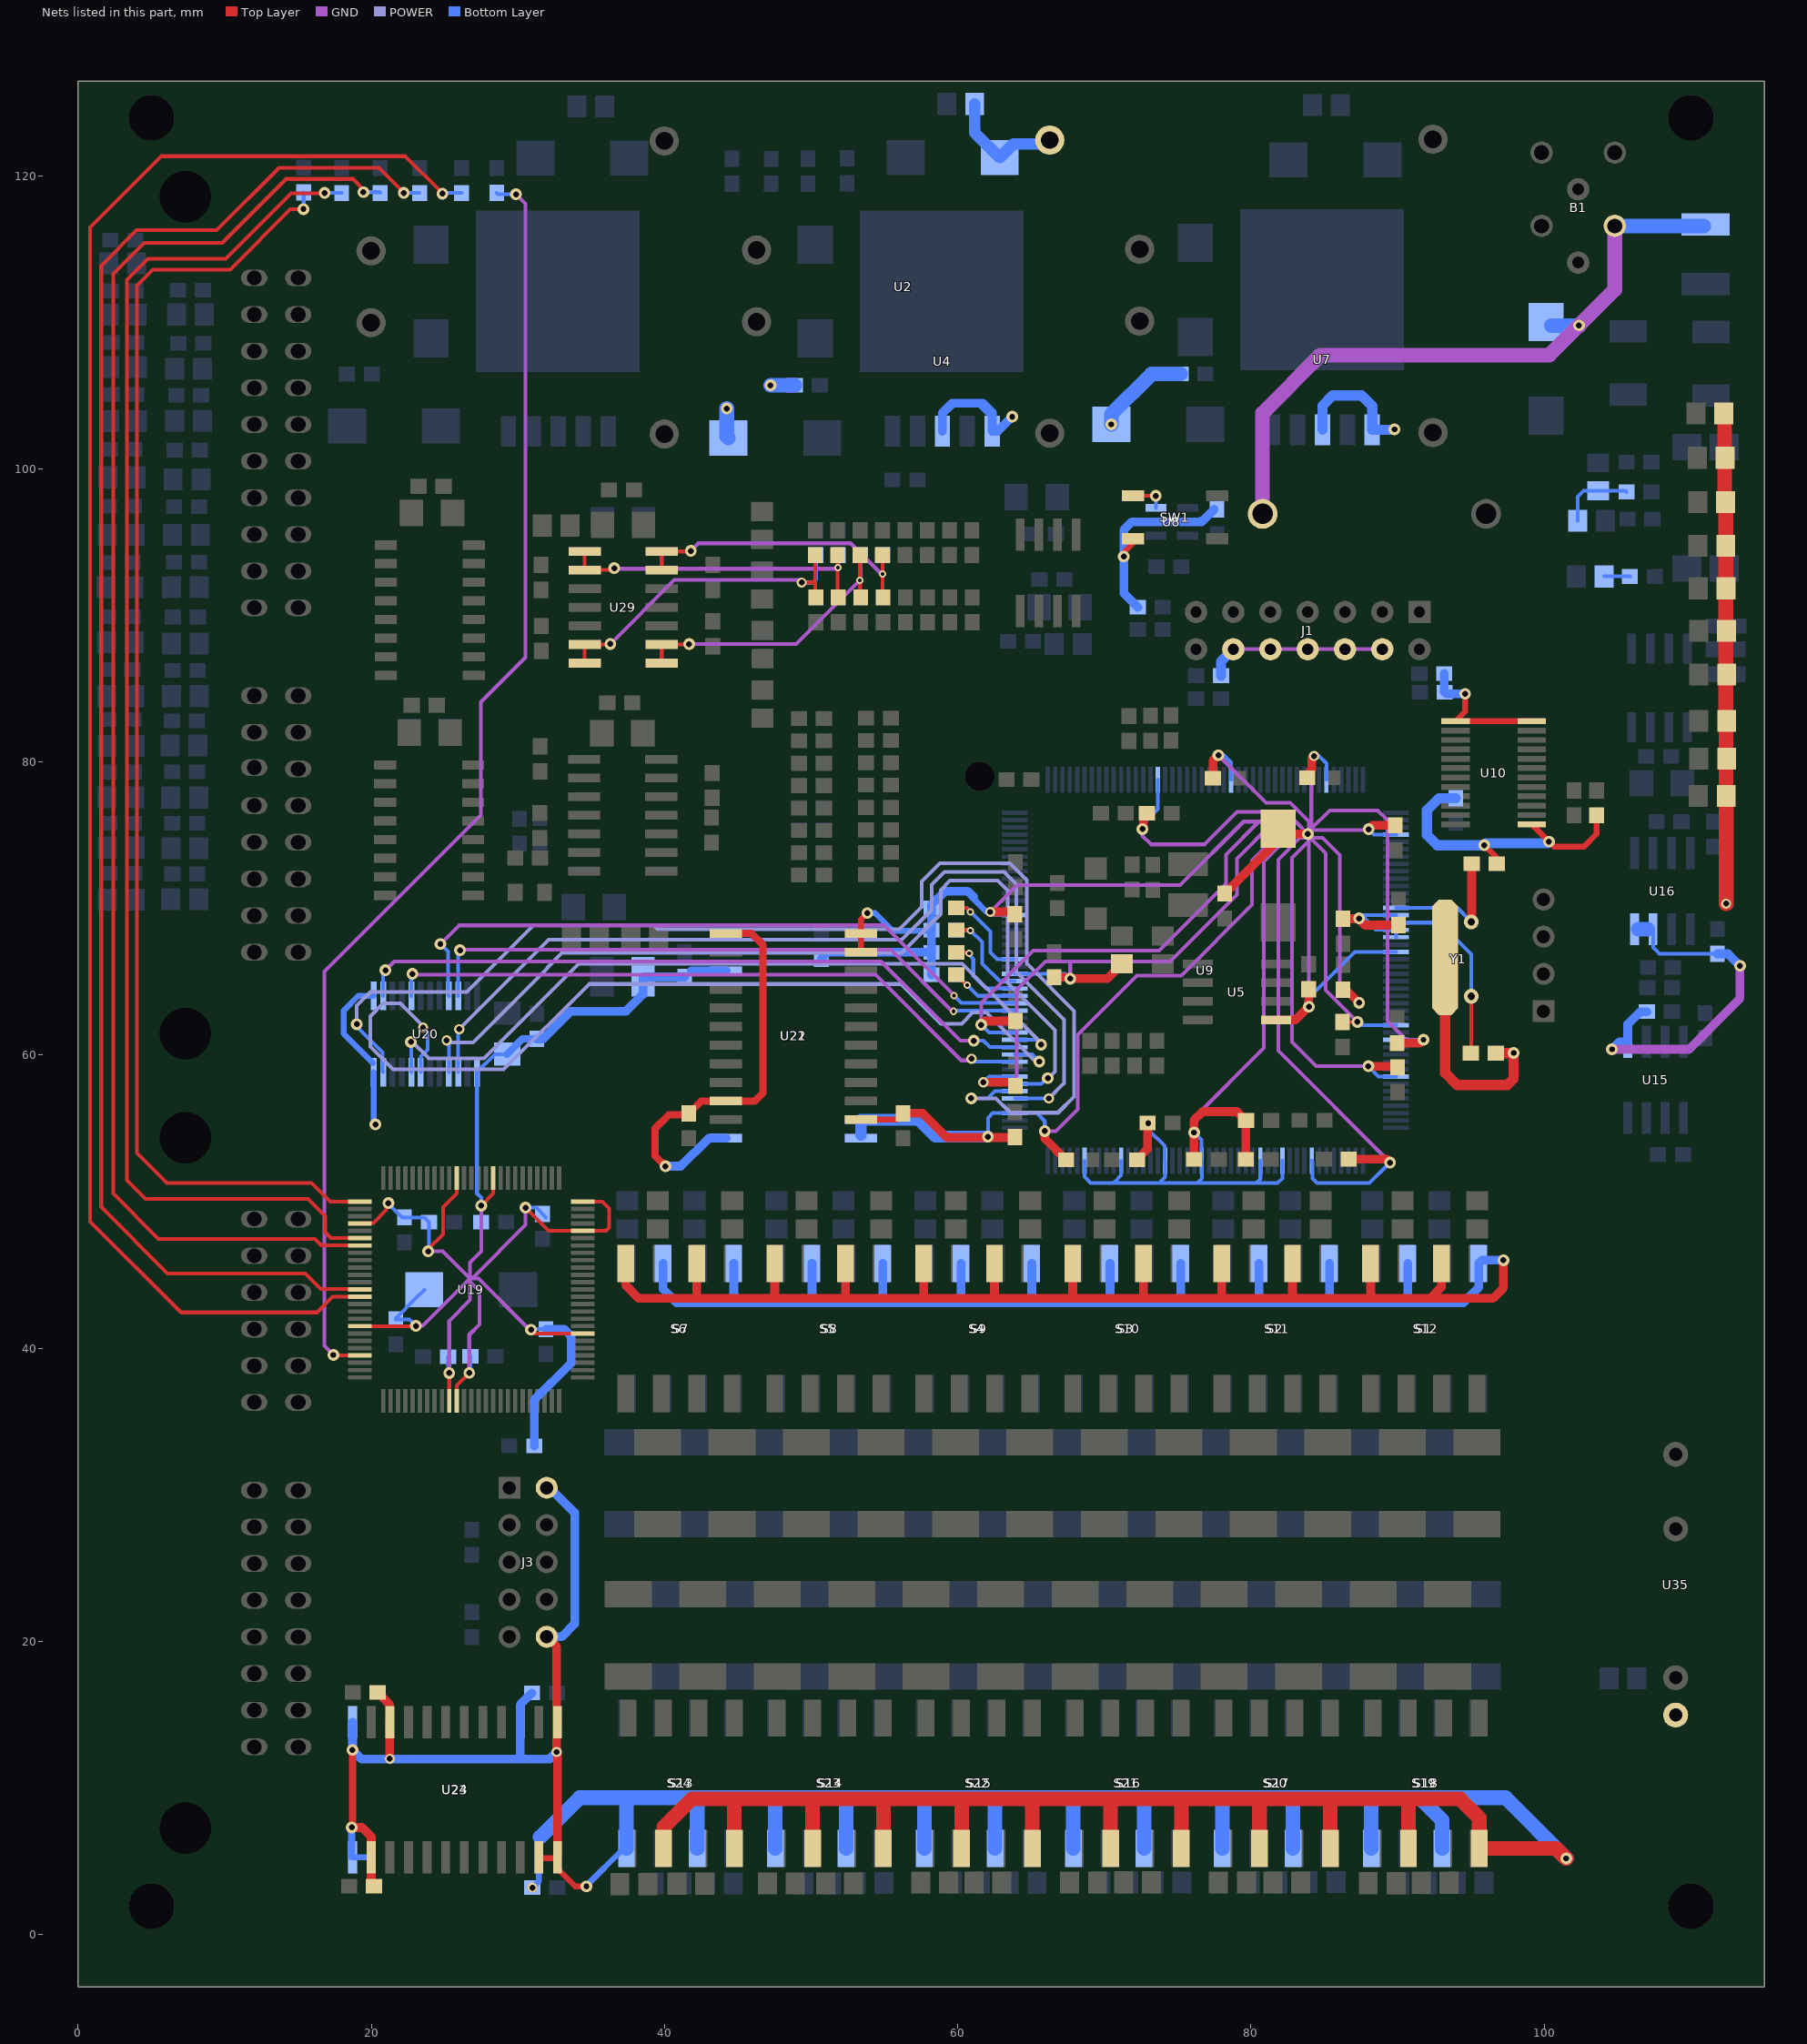
[diagram p0: the nets of this part, all layers, seen from the top]
# Altium PCB MISC86180.PCBDOC (part 7 of 9)
Units mm, origin at the board's own origin, x right, y up, seen from the top; angles counter-clockwise.
Board outline 115 x 130 mm, 4 copper layers (Top Layer, GND, POWER, Bottom Layer); 475 components, 355 nets, 1755 pads, 459 vias.

## Via types
v1: diameter 0.8, hole 0.4, Top Layer to Bottom Layer, 339 vias
v2: diameter 0.7, hole 0.4, Top Layer to Bottom Layer, 83 vias
v3: diameter 0.5, hole 0.254, Top Layer to Bottom Layer, 37 vias

## Nets (pads, with @x,y where several pads share a name; then routed paths per layer and width w, separated by ;. In a path a pad name is that pad's centre, name@x,y a point inside that pad or via, vN(x,y) a via of type N, cw(c..) or ccw(c..) an arc to the next point about the centre after c; other vN are vias at no path point) (continued)
GNDD: C6.2 C7.1 C11.2 C12.1 C13.2 C14.1 C17.2 C18.1 C19.1 C20.1 C21.1 C22.1 C23.1 C24.1 C25.1 C26.1 C27.1 C28.1 C29.1 C30.1 C31.1 C32.1 C33.1 C34.1 C35.1 C36.1 C37.1 C38.1 C39.1 C40.1 C41.1 C42.1 C52.1 C53.1 C54.1 C55.1 C56.1 C57.1 C67.1 C68.1 C81.2 C82.1 C83.1 C84.1 C85.1 C86.1 C87.1 C88.1 C89.1 C90.1 C91.1 C92.1 C93.1 C94.1 C95.1 C96.1 C97.1 C98.1 C99.1 D1.2 D2.2 D3.2 D4.2 D5.2 D6.2 D7.2 D8.2 D9.2 D10.2 J1.4 J1.6 J1.8 J1.10 J1.12 J3.2 J3.10 L2.1 R4.1 R5.1 R14.1 R83.1 R87.2 R89.2 R91.2 R93.2 S1.2 S1.4 S2.2 S2.4 S3.2 S3.4 S4.2 S4.4 S5.2 S5.4 S6.2 S6.4 S7.2 S7.4 S8.2 S8.4 S9.2 S9.4 S10.2 S10.4 S11.2 S11.4 S12.2 S12.4 S13.2 S13.4 S14.2 S14.4 S15.2 S15.4 S16.2 S16.4 S17.2 S17.4 S18.2 S18.4 S19.2 S19.4 S20.2 S20.4 S21.2 S21.4 S22.2 S22.4 S23.2 S23.4 S24.2 S24.4 SW1.2 U2.4 U4.1 U4.3 U5.1 U7.1 U7.3 U8.2 U9.3 U9.8 U9.14 U9.22 U9.30 U9.60 U9.70 U9.83 U9.92 U9.103 U9.105 U9.106 U9.108 U9.118 U9.120 U9.125 U9.140 U9.144 U9.147 U9.155 U9.160 U9.166 U9.171 U10.1 U10.12 U10.13 U15.5 U16.3 U16.4 U19.10 U19.11 U19.32 U19.46 U19.50 U19.60 U19.65 U19.79 U19.93 U20.1 U20.12 U20.13 U21.2 U21.11 U21.12 U21.13 U21.22 U22.2 U22.11 U22.12 U22.13 U22.22 U23.2 U23.11 U23.12 U23.13 U23.22 U24.2 U24.11 U24.12 U24.13 U24.22 U35.1 Y1.3 | length 1278
  Top Layer w0.254: U19.93@19.216,41.514 v1@23.024,41.514 ; U19.79@19.216,48.514 19.261,48.559 20.142,48.559 21.02,49.437 21.02,49.79 21.14,49.91 v1(21.17,49.91) ; U23.2@19.98,5.283 U23.2@19.989,5.292 ; U23.22@21.259,14.492 21.259,15.681 21.268,15.69 21.259,15.699 ; v1(23.88,46.62) 23.88,46.77 24.89,47.78 24.89,49.63 25.816,50.556 U19.65@25.816,51.614 ; U19.10@25.316,36.414 v1(25.316,38.314) ; U19.11@25.816,36.414 25.816,37.456 v1(26.68,38.32) ; v1(27.49,49.73) 28.316,50.556 U19.60@28.316,51.614 ; v1(30.52,49.59) 32.096,48.014 U19.46@34.416,48.014 35.994,48.014 36.21,48.23 36.21,49.55 35.746,50.014 U19.50@34.416,50.014 ; v1(30.89,41.27) 31.146,41.014 U19.32@34.416,41.014 ; S13.4@44.763,5.884 44.763,8.343 44.84,8.42 ; 52.343,43.427 52.343,43.56 ; 57.677,43.467 57.677,43.68 ; v1(61.59,62.07) v1@61.705,62.185 ; C42.1@63.878,54.41 C42.1@63.908,54.41 ; v1@67.58,65.31 v1(67.67,65.22) ; v1(72.59,75.42) v1@72.66,75.49 ; C20.1@72.94,55.37 C20.1@72.94,55.372 ; 82.823,43.467 82.823,43.53 ; v2@84.19,80.31 v2(84.29,80.41) ; C23.1@86.232,62.26 v1@87.24,62.26 ; v1(88.02,75.41) v1@88.11,75.5 ; 88.157,43.453 88.157,43.77 ; C34.1@89.922,59.24 C34.1@89.982,59.18 ; S18.2@90.71,5.911 S18.2@90.737,5.884 ; v1@91.53,60.82 v1(91.76,61.05) ; 94.97,8.25 95.563,7.657
  Top Layer w0.4: U23.11@31.37,5.21 U23.12@32.64,5.21 ; U23.12@32.695,5.28 32.695,4.495 33.9,3.29 v1(34.67,3.29) ; U22.2@53.392,55.599 55.841,55.599 C96.1@56.272,56.03 ; U22.11@53.392,67.029 U22.12@53.392,68.299 53.392,69.252 v1(53.83,69.69) ; v1(71.32,94.02) 71.32,94.29 71.939,94.909 SW1.2@71.939,95.233 ; v1(94.6,84.65) 94.6,83.432 U10.13@93.946,82.778 U10.12@99.146,82.778 ; v1(95.9,74.32) 96.75,73.47 C55.1@96.75,73.062 ; U10.1@99.146,75.738 v1(100.322,74.562) 100.675,74.21 102.69,74.21 103.568,75.088 R14.1@103.568,76.36
  Top Layer w0.5: v1@18.71,7.36 v1(18.71,12.6) ; v1(40.06,52.42) 39.36,53.12 39.36,54.99 40.29,55.92 41.552,55.92 C92.1@41.662,56.03 42.501,56.869 U22.22@44.192,56.869 46.159,56.869 46.7,57.41 46.7,67.53 45.931,68.299 U22.13@44.192,68.299
  Top Layer w0.6: v1@18.71,7.36 18.76,7.31 19.36,7.31 19.989,6.681 U23.2@19.989,5.292 ; U23.2@19.995,5.28 19.995,3.493 C98.1@20.18,3.308 ; C94.1@20.43,16.528 21.259,15.699 21.259,15.681 ; v2(21.26,12) U23.22@21.259,14.492 ; J3.10@31.965,20.325 32.64,19.65 v2(32.64,12.46) ; U23.12@32.689,5.292 v2@32.689,12.46 ; U23.13@32.689,14.48 U23.13@32.689,14.492 ; S6.4@37.357,45.792 37.357,44.283 38.233,43.407 42.183,43.407 ; S6.2@42.183,45.792 42.183,43.407 ; 47.517,43.427 S5.4@47.517,45.792 ; 52.343,43.56 S5.2@52.343,45.792 ; C96.1@56.272,56.03 57.6,56.03 59.25,54.38 C42.1@63.878,54.38 ; 57.677,43.68 S4.4@57.677,45.792 ; v1@61.705,62.185 61.844,62.324 C41.1@63.918,62.324 ; v2(61.74,58.15) 63.688,58.15 C27.1@63.928,57.91 ; v2(62.22,69.77) 63.724,69.77 C36.1@63.882,69.612 ; 62.503,43.53 S4.2@62.503,45.792 ; v1(65.93,54.82) 65.93,54.312 C25.1@67.38,52.862 ; C37.1@66.568,65.31 v1@67.58,65.31 ; v1(67.67,65.22) 70.189,65.22 R4.1@71.188,66.219 ; 67.837,43.474 S3.4@67.837,45.792 ; C30.1@72.22,52.868 72.94,53.588 C20.1@72.94,55.37 ; v1@72.66,75.49 C38.1@72.66,76.472 ; 72.663,43.413 S3.2@72.663,45.792 ; C31.1@76.1,52.902 76.1,55.55 76.7,56.15 79.052,56.15 C22.1@79.66,55.542 79.64,55.522 C32.1@79.64,52.902 ; C28.1@77.4,78.902 77.4,80.09 v1(77.77,80.46) ; 77.997,43.417 S2.4@77.997,45.792 ; C14.1@78.212,71.02 82.277,75.085 v1(83.875,75.085) ; U5.1@81.713,62.4 83.006,62.4 83.928,63.322 C26.1@83.928,64.5 ; 82.823,43.53 S2.2@82.823,45.792 ; C29.1@83.84,78.922 83.84,79.17 84.14,79.47 84.14,80.26 v2@84.19,80.31 ; C40.1@86.258,64.47 86.47,64.47 v1(87.37,63.57) ; C24.1@86.262,69.3 87.34,69.3 87.77,68.87 C39.1@90.058,68.87 ; C33.1@86.66,52.908 89.242,52.908 v1(89.48,52.67) ; v1(88,59.24) C34.1@89.922,59.24 ; v1@88.11,75.5 88.29,75.68 C21.1@89.832,75.68 ; 88.157,43.77 S1.4@88.157,45.792 ; C35.1@89.968,60.82 v1@91.53,60.82 ; S1.2@92.983,45.173 92.983,44.173 92.217,43.407 ; v1(97.21,46.01) 97.21,44.12 96.497,43.407 92.217,43.407 ; 42.183,43.407 92.217,43.407
  Top Layer w0.7: Y1.3@93.242,66.677 93.242,58.778 94.06,57.96 97.48,57.96 97.906,58.386 v1(97.906,60.15) 97.895,60.138 C56.1@96.69,60.138
  Top Layer w1: S13.2@39.937,5.884 39.937,7.337 41.86,9.26 94.266,9.26 95.563,7.963 95.563,7.657 S18.4@95.563,5.884 100.806,5.884 v1@101.49,5.2 ; 44.76,9.05 S13.4@44.763,5.884 ; S14.2@50.097,5.884 50.097,9.05 ; S14.4@54.923,5.884 54.923,8.99 ; S15.2@60.257,5.884 60.257,8.95 ; S15.4@65.083,5.884 65.083,9.17 ; S16.2@70.417,5.884 70.417,9.07 ; S16.4@75.243,5.884 75.243,8.89 ; S17.2@80.577,5.884 80.577,9.04 ; S17.4@85.403,5.884 85.403,9.03 ; S18.2@90.737,5.884 90.737,8.9 ; D7.2@112.31,97.73 D5.2@112.31,103.77 ; D2.2@112.38,82.78 D7.2@112.38,97.72 ; v2(112.4,70.33) 112.409,70.339 D3.2@112.409,77.682 ; D3.2@112.4,77.83 D2.2@112.4,82.78
  GND w0.254: v1(23.04,41.53) 23.51,41.53 26.73,44.75 ; v1(23.88,46.62) 24.86,46.62 26.73,44.75 ; v1(25.316,38.314) 25.316,41.886 26.73,43.3 26.73,44.54 ; v1(26.68,38.32) 26.68,40.93 27.39,41.64 27.39,43.88 26.73,44.54 ; v1(27.49,49.73) 27.49,46.61 26.73,45.85 26.73,44.85 ; v1(30.52,49.59) 30.52,48.41 26.96,44.85 26.73,44.85 ; v1(30.89,41.27) 30.79,41.27 27.31,44.75 26.83,44.75 ; v1(61.59,62.07) 61.59,63.57 65.15,67.13 73.72,67.13 78.29,71.7 78.29,73.69 80.53,75.93 ; v2(61.74,58.15) 63.58,58.15 64.03,58.6 64.03,64.46 65.97,66.4 67.71,66.4 ; v2(62.22,69.77) 64.04,71.59 75.15,71.59 79.49,75.93 80.53,75.93 ; v1(65.93,54.82) 66.68,54.82 68.17,56.31 68.17,61.38 72.22,65.43 75.25,65.43 80.075,70.255 80.075,73.285 81.875,75.085 82.765,75.085 ; v1(67.67,65.22) 67.67,66.36 67.71,66.4 ; v1(72.59,75.42) 72.59,74.96 73.17,74.38 76.84,74.38 79.05,76.59 82.37,76.59 83.03,75.93 ; v1(76.12,54.72) 76.12,55.73 80.88,60.49 80.88,73.2 82.765,75.085 ; v1(77.77,80.46) 81.02,77.21 82.68,77.21 83.95,75.94 v1@83.95,75.01 ; J1.12@78.786,87.693 J1.10@81.326,87.693 J1.8@83.866,87.693 J1.6@86.406,87.693 J1.4@88.946,87.693 ; v1(83.95,63.3) 83.95,74.6 ; 84.29,75.35 87.96,75.35 v1(88.02,75.41) ; v2(84.29,80.41) 84.11,80.23 84.11,75.44 ; v1(87.25,62.27) 85.09,64.43 85.09,73.78 84.11,74.76 ; v1(87.37,63.57) 86.05,64.89 86.05,73.65 84.87,74.83 84.18,74.83 84.11,74.76 ; v1(88,59.24) 84.45,59.24 82.8,60.89 82.8,73.45 83.95,74.6 ; v1(89.48,52.67) 81.85,60.3 81.85,73.34 83.33,74.82 v1@83.95,74.82 ; v1(91.76,61.05) 90.59,61.05 89.31,62.33 89.31,76.03 88.64,76.7 85.37,76.7 84.11,75.44 ; 26.73,44.54 26.73,44.75 ; 26.73,44.75 26.73,44.85 ; 26.73,44.75 26.83,44.75 ; 26.73,44.85 26.83,44.75 ; 67.71,66.4 74.47,66.4 79.03,70.96 79.03,73.4 81.56,75.93 ; 80.53,75.93 81.56,75.93 ; 81.56,75.93 83.03,75.93 ; 82.765,75.085 v1(83.875,75.085) ; 83.03,75.93 v1(83.875,75.085) ; v1(83.875,75.085) v1@83.95,75.01 ; 83.95,74.6 v1@83.95,74.82 ; 83.95,74.6 84.11,74.76 ; v1@83.95,74.82 v1@83.95,75.01 ; v1@83.95,75.01 84.11,75.17 84.11,75.44
  GND w0.6: v1(104.61,60.4) 109.87,60.4 113.35,63.88 v1(113.35,66.09)
  Bottom Layer w0.254: v1(21.17,49.91) 21.17,49.85 22.092,48.928 C87.1@22.262,48.928 23.61,48.928 C89.1@23.934,48.604 23.934,46.674 v1(23.88,46.62) ; C86.1@21.658,41.97 22.6,41.97 v1(23.04,41.53) ; C86.1@21.658,42.044 23.04,43.426 C81.2@23.61,43.996 ; C88.1@25.23,39.422 25.23,38.4 v1(25.316,38.314) ; v1(26.68,38.32) 26.76,38.4 C83.1@26.76,39.448 ; C82.1@27.49,48.604 v1(27.49,49.73) 27.49,50.29 27.208,50.572 U20.1@27.208,58.842 28.433,60.067 C91.1@29.256,60.067 ; v1(30.52,49.59) 31.252,49.59 C84.1@31.914,48.928 ; v1@30.928,41.308 C85.1@31.914,41.308 ; 37.39,9.06 S24.4@37.397,6.069 ; C93.1@41.377,65.335 C93.1@41.382,65.33 C93.1@41.811,65.759 ; 50.057,43.217 50.057,43.45 ; R89.2@58.144,67.006 58.121,67.029 R89.2@58.177,67.029 ; R91.2@58.15,68.58 R91.2@58.2,68.53 ; R89.2@58.2,67.006 R89.2@58.2,67.029 ; U4.3@58.947,102.565 58.947,103.537 59.79,104.38 61.37,104.38 62.347,103.403 U4.1@62.347,102.565 ; 60.217,43.227 60.217,43.39 ; 61.151,122.933 61.252,122.832 ; v1(61.59,62.07) 62.117,61.543 U9.14@63.889,61.543 ; v2(61.74,58.15) 62.133,58.543 U9.8@63.889,58.543 ; v1@62.06,54.44 62.06,55.72 62.383,56.043 U9.3@63.889,56.043 65.377,56.043 65.93,55.49 v1(65.93,54.82) ; v2(62.22,69.77) 62.447,69.543 U9.30@63.889,69.543 ; U9.22@63.889,65.543 67.347,65.543 v1(67.67,65.22) ; 65.043,43.223 65.043,43.34 ; U2.4@66.001,122.159 U2.4@66.271,122.428 ; U9.171@68.639,52.793 68.639,51.7 69.065,51.275 ; 69.08,51.28 80.35,51.28 80.639,51.569 U9.147@80.639,52.793 ; 70.377,43.123 70.377,43.43 ; 70.71,51.37 71.139,51.799 U9.166@71.139,52.793 ; v1(72.59,75.42) 72.59,75.732 73.639,76.781 U9.60@73.639,78.793 ; S21.2@72.69,5.897 S21.2@72.703,5.884 ; v1(72.99,55.37) 72.99,54.913 74.094,53.809 74.094,52.839 U9.160@74.139,52.793 74.139,51.679 73.85,51.39 ; 75.203,43.127 75.203,43.43 ; v1(76.12,54.72) 76.61,54.23 U9.155@76.61,52.823 ; 76.34,51.29 76.639,51.589 U9.155@76.639,52.793 ; v1(77.77,80.46) 78.15,80.46 78.639,79.971 U9.70@78.639,78.793 ; 80.34,51.27 81.81,51.27 82.139,51.599 U9.144@82.139,52.793 ; v1@83.93,63.32 83.93,63.893 87.08,67.043 U9.108@89.889,67.043 ; U9.140@84.139,52.793 84.18,52.753 84.18,51.59 84.5,51.27 88.08,51.27 v1(89.48,52.67) ; v2(84.29,80.41) 84.628,80.41 85.139,79.899 U9.83@85.139,78.793 ; 85.363,43.197 85.363,43.3 ; v1(87.25,62.27) 87.477,62.043 U9.118@89.889,62.043 ; v1(88,59.24) 88.697,58.543 U9.125@89.889,58.543 ; v1(88.02,75.41) 88.387,75.043 U9.92@89.889,75.043 ; U9.120@89.889,61.043 v1@91.753,61.043 ; U9.106@89.889,68.043 U9.105@89.889,68.543 89.858,68.575 88.505,68.575 87.75,69.33 v1(87.37,69.33) 87.583,69.543 U9.103@89.889,69.543 ; S19.2@93.023,5.884 S19.2@93.023,7.147 ; R5.1@93.18,86.032 R5.1@93.21,86.002 ; U16.3@107.423,68.591 107.423,67.337 107.85,66.91 C68.1@111.802,66.91
  Bottom Layer w0.4: U24.12@18.719,5.292 U24.11@19.989,5.292 ; U20.12@20.105,59.465 18.11,61.46 18.11,63.04 19.112,64.042 U20.13@20.168,64.042 ; U20.12@20.168,58.842 20.168,55.382 v1(20.28,55.27) ; v2(30.98,3.208) 31.419,3.647 U24.2@31.419,5.292 31.419,6.359 31.419,6.479 ; v1(34.67,3.29) 34.67,3.34 S24.4@37.2,5.87 ; v1(53.83,69.69) 54.35,69.69 55.55,68.49 58.16,68.49 R91.2@58.2,68.53 ; 61.07,70.666 v2@61.966,69.77
  Bottom Layer w0.5: U24.12@18.67,5.341 v1(18.67,7.32) ; C91.1@29.256,60.067 30.305,61.116 C90.1@31.288,61.116 ; U24.2@31.38,6.32 31.419,6.359 31.479,6.419
  Bottom Layer w0.6: v1@18.719,12.591 19.32,11.99 32.17,11.99 v2(32.64,12.46) ; v1@18.719,12.6 U24.13@18.719,14.492 ; 30.149,12.029 U24.22@30.149,14.492 30.149,15.677 C95.1@30.96,16.488 ; R83.1@31.11,33.332 31.11,36.47 33.63,38.99 33.63,40.83 33.152,41.308 C85.1@31.914,41.308 ; C90.1@31.288,61.116 31.726,61.116 33.61,63 37.38,63 38.525,64.145 L2.1@38.525,65.335 ; J3.10@31.965,20.325 32.985,20.325 33.87,21.21 33.87,28.78 32.165,30.485 J3.2@31.965,30.485 ; L2.1@38.525,65.136 L2.1@38.525,65.335 ; S7.2@39.897,45.792 39.897,44.033 40.81,43.12 94.49,43.12 95.523,44.153 S12.4@95.523,45.792 95.741,46.01 v1(97.21,46.01) ; v1(40.06,52.42) 41.1,52.42 43.009,54.329 U21.13@44.192,54.329 ; C93.1@41.377,65.335 L2.1@38.525,65.335 ; C93.1@41.811,65.759 U21.22@44.192,65.759 ; 44.723,43.167 S7.4@44.723,45.792 ; 50.057,43.45 S8.2@50.057,45.792 ; C97.1@50.692,66.58 51.141,67.029 U21.2@53.392,67.029 R89.2@58.121,67.029 ; 54.883,43.257 S8.4@54.883,45.792 ; R87.2@58.2,65.482 R89.2@58.2,67.006 R91.2@58.2,68.53 R93.2@58.2,70.054 58.2,70.252 59.138,71.19 60.662,71.19 61.07,70.782 ; U4.3@58.947,102.565 58.947,103.807 59.62,104.48 61.71,104.48 62.347,103.843 U4.1@62.347,102.565 62.725,102.565 v1(63.71,103.55) ; 60.217,43.39 S9.2@60.217,45.792 ; 65.043,43.34 S9.4@65.043,45.792 ; 70.377,43.43 S10.2@70.377,45.792 ; C53.1@72.272,90.556 71.32,91.508 v1(71.32,94.02) 71.32,95.82 71.885,96.385 U8.2@73.512,96.385 76.633,96.385 ; 75.203,43.43 S10.4@75.203,45.792 ; 76.633,96.46 76.708,96.46 C19.1@77.474,97.226 ; 80.537,43.153 S11.2@80.537,45.792 ; 85.363,43.3 S11.4@85.363,45.792 ; 90.697,43.173 S12.2@90.697,45.792 ; R5.1@93.18,86.032 93.18,84.792 C52.1@93.21,84.762 93.322,84.65 v1(94.6,84.65) ; v1(104.61,60.4) 105.123,60.913 U15.5@105.691,60.913 105.691,62.111 106.548,62.968 C67.1@107,62.968 ; C68.1@111.802,66.91 112.53,66.91 v1(113.35,66.09)
  Bottom Layer w0.7: C54.1@77.95,85.892 77.95,86.857 J1.12@78.786,87.693 ; U7.3@84.867,102.665 84.867,104.307 85.56,105 87.54,105 88.267,104.273 U7.1@88.267,102.665 89.755,102.665 v1(89.78,102.69) ; C57.1@93.968,77.53 92.81,77.53 92,76.72 92,75.01 92.69,74.32 v1(95.9,74.32) 96.03,74.45 100.21,74.45 v1(100.322,74.562)
  Bottom Layer w0.8: U21.12@53.392,54.55 U21.11@53.392,55.44 ; U21.11@53.392,55.599 57.301,55.599 58.46,54.44 v1(62.05,54.44) v1@62.06,54.44 ; 61.151,122.933 C7.1@61.151,124.892 ; 61.252,122.832 C6.2@62.856,121.228 63.786,122.159 U2.4@66.001,122.159
  Bottom Layer w1: 31.518,6.652 34.206,9.34 91.5,9.34 ; 37.39,9.06 S24.4@37.397,5.884 S24.4@37.397,6.069 ; S24.2@42.223,5.884 42.223,9.13 ; v1(44.24,104.11) 44.24,102.216 C11.2@44.354,102.102 ; v1(47.23,105.69) 47.232,105.688 C12.1@48.88,105.688 ; S23.4@47.557,5.884 47.557,8.91 ; S23.2@52.383,5.884 52.383,9.03 ; S22.4@57.717,5.884 57.717,9.14 ; S22.2@62.543,5.884 62.543,9.14 ; S21.4@67.877,5.884 67.877,9.1 ; v1(70.464,103.032) 70.464,103.722 73.21,106.468 C18.1@75.19,106.468 ; S21.2@72.703,5.884 72.703,9.05 ; S20.4@78.037,5.884 78.037,9.1 ; S20.2@82.863,5.884 82.863,9.14 ; S19.4@88.197,5.884 88.197,9.05 ; S19.2@93.023,5.884 93.023,7.147 93.023,7.817 92.303,8.537 91.5,9.34 ; 97.36,9.34 91.5,9.34 ; 97.455,9.245 v1(101.5,5.2) ; U16.4@106.41,68.591 107.049,68.591
GPIO0: U9.5 U20.3 | length 65.5
  POWER w0.254: v2(25.99,61.77) 32.09,67.87 56.17,67.87 58.21,69.91 58.21,71.62 59.09,72.5 63.15,72.5 63.99,71.66 63.99,65.67 67.25,62.41 67.25,58.09 v2(66.21,57.05)
  Bottom Layer w0.254: U20.3@25.928,58.842 25.928,61.708 v2(25.99,61.77) ; U9.5@63.889,57.043 66.203,57.043 v2(66.21,57.05)
GPIO1: U9.6 U20.11 | length 83.9
  POWER w0.254: v1(19.01,62.11) 19.01,63.38 19.93,64.3 26.5,64.3 31.06,68.86 39.251,68.86 39.531,68.58 56.02,68.58 57.547,70.107 57.547,71.857 58.77,73.08 63.56,73.08 64.7,71.94 64.7,66.25 67.94,63.01 67.94,57.18 66.83,56.07 63.58,56.07 62.59,57.06 v1(60.91,57.06)
  Bottom Layer w0.254: v1(19.01,62.11) 19.01,61.94 20.765,60.185 20.765,58.884 U20.11@20.808,58.842 ; v1(60.91,57.06) 62.05,57.06 62.533,57.543 U9.6@63.889,57.543
GPIO2: U9.7 U20.4 | length 63.3
  POWER w0.254: v2@25.07,61.05 25.07,60.91 25.11,60.87 26.93,60.87 31.99,65.93 31.99,65.97 33,66.98 56.18,66.98 58.83,69.63 58.83,71.26 59.47,71.9 62.71,71.9 63.39,71.22 63.39,64.93 66.62,61.7 66.62,58.88 v1@66.17,58.43
  Bottom Layer w0.254: v2@25.07,61.05 25.07,60.99 25.288,60.772 U20.4@25.288,58.842 ; U9.7@63.889,58.043 65.693,58.043 v1@66.08,58.43
  other v1: 66.14,58.43
  other v2: 25.14,61
GPIO3: U9.10 U20.17 | length 45.2
  GND w0.254: v1(22.8,65.54) 22.8,65.52 22.83,65.49 54.39,65.49 60.24,59.64 60.83,59.64 v2(60.94,59.75)
  Bottom Layer w0.254: U20.17@22.728,64.042 22.728,65.498 22.77,65.54 v1(22.8,65.54) ; v2(60.94,59.75) 61.14,59.55 63.883,59.55 U9.10@63.889,59.543
GPIO4: U9.11 U20.7 | length 63.4
  POWER w0.254: v2@23.53,62.03 23.47,62.03 21.97,63.53 20.81,63.53 19.93,62.65 19.93,60.59 21.49,59.03 29.03,59.03 34.85,64.85 56.13,64.85 58.84,62.14 60.26,62.14 61.02,62.9 61.95,62.9 65.29,59.56 v1(65.56,59.56)
  Bottom Layer w0.254: U20.7@23.368,58.842 23.368,59.898 23.83,60.36 23.83,61.59 v2(23.53,61.89) ; U9.11@63.889,60.043 65.077,60.043 v1(65.56,59.56)
GPIO5: U9.12 U20.14 | length 47.5
  GND w0.254: v1(20.96,65.79) 21.56,66.39 54.76,66.39 60.17,60.98 v1(61.09,60.98)
  Bottom Layer w0.254: U20.14@20.808,64.042 20.808,65.883 20.835,65.91 20.84,65.91 v1(20.96,65.79) ; v1@61.22,60.97 61.24,60.99 61.74,60.99 62.187,60.543 U9.12@63.889,60.543
GPIO6: U9.13 U20.8 | length 52.5
  POWER w0.254: v1(22.7,60.9) 22.8,60.9 23.92,59.78 27.69,59.78 34.14,66.23 60.3,66.23 65.68,60.85 v1(65.68,60.72)
  Bottom Layer w0.254: v1(22.7,60.9) 22.728,60.872 U20.8@22.728,58.842 ; U9.13@63.889,61.043 65.357,61.043 v1(65.68,60.72)
GPIO8: U9.17 U20.22 | length 42.8
  GND w0.254: v1(26.05,67.16) 26.08,67.19 55.42,67.19 59.63,62.98 v3@59.7,62.98
  Bottom Layer w0.254: U20.22@25.928,64.042 25.928,67.038 v1(26.05,67.16) ; v3@59.67,63.04 60.56,63.04 60.563,63.043 U9.17@63.889,63.043
  other v3: 59.71,62.99
GPIO9: U9.18 U20.21 | length 45.8
  GND w0.254: v1(24.71,67.58) 25.983,68.853 54.987,68.853 v3@59.83,64.01
  Bottom Layer w0.254: v1(24.71,67.58) 25.23,67.06 25.23,64.099 U20.21@25.288,64.042 ; v3@59.75,64.05 60.23,63.57 63.863,63.57 U9.18@63.889,63.543
  other v3: 59.75,64.07
GPIO10: R86.2 R87.1 U9.19 | length 5.8
  Top Layer w0.254: R86.2@59.9,65.482 60.602,64.78 v3(60.64,64.78)
  Bottom Layer w0.254: R87.1@60.02,65.362 R87.1@59.9,65.482 59.938,65.482 61.377,64.043 U9.19@63.889,64.043
GPIO11: R88.2 R89.1 U9.20 | length 6.6
  Top Layer w0.254: R88.2@59.89,67.016 R88.2@59.9,67.006 60.714,67.006 v3(60.78,66.94)
  Bottom Layer w0.254: R89.1@59.9,67.006 60.594,67.006 61.06,66.54 61.06,65.39 61.9,64.55 63.883,64.55 U9.20@63.889,64.543
GPIO12: R90.2 R91.1 U9.21 | length 7.2
  Top Layer w0.254: R90.2@59.89,68.54 R90.2@59.9,68.53 60.82,68.53 v3(60.85,68.5)
  Bottom Layer w0.254: R91.1@59.9,68.53 v3@60.84,68.53 ; v3@60.86,68.51 61.66,67.71 61.66,66.24 62.857,65.043 U9.21@63.889,65.043
GPIO13: R92.2 R93.1 U9.24 | length 7.4
  Top Layer w0.254: R92.2@59.9,70.054 60.576,70.054 v3(60.86,69.77)
  Bottom Layer w0.254: R93.1@59.85,70.11 59.85,70.104 R93.1@59.9,70.054 60.596,70.054 62.22,68.43 62.22,67.01 62.687,66.543 U9.24@63.889,66.543
LED1: R98.1 U19.76 | length 90.4
  Top Layer w0.254: v1@15.34,117.71 14.48,117.71 10.36,113.59 5.1,113.59 4.013,112.503 4.013,53.337 6.07,51.28 15.93,51.28 17.196,50.014 U19.76@19.216,50.014
  Bottom Layer w0.254: v1(15.37,117.71) 15.386,117.726 R98.1@15.386,118.854
LED2: R99.1 U19.81 | length 96.8
  Top Layer w0.254: v1@16.84,118.86 16.78,118.8 14.54,118.8 10.07,114.33 4.76,114.33 3.32,112.89 3.32,51.46 4.6,50.18 15.669,50.18 16.85,48.999 16.85,47.91 17.246,47.514 U19.81@19.216,47.514
  Bottom Layer w0.254: v1(16.81,118.82) 17.966,118.82 R99.1@17.972,118.814
LED3: R100.1 U19.82 | length 102.5
  Top Layer w0.254: U19.82@19.216,47.014 16.596,47.014 16.14,47.47 5.48,47.47 2.39,50.56 2.39,113.29 4.51,115.41 9.83,115.41 14.19,119.77 18.74,119.77 v1@19.645,118.865
  Bottom Layer w0.254: v1(19.46,118.87) 20.542,118.87 R100.1@20.598,118.814
LED4: R101.1 U19.88 | length 109.4
  Top Layer w0.254: U19.88@19.216,44.014 19.171,44.059 16.543,44.059 15.492,45.11 6.1,45.11 1.58,49.63 1.58,113.87 3.98,116.27 9.45,116.27 13.71,120.53 20.52,120.53 v1@22.22,118.83
  Bottom Layer w0.254: v1(22.21,118.82) 22.216,118.814 R101.1@23.294,118.814 R101.1@23.288,118.82
LED5: R102.1 U19.89 | length 117.6
  Top Layer w0.254: U19.89@19.216,43.514 17.354,43.514 16.29,42.45 7.02,42.45 0.82,48.65 0.82,116.47 5.67,121.32 22.33,121.32 v1@24.885,118.765
  Bottom Layer w0.254: v1@24.894,118.814 R102.1@26.15,118.814
  other v1: 24.85,118.77
LED6: R103.1 U19.97 | length 88.6
  Top Layer w0.254: v1(17.41,39.55) 17.446,39.514 U19.97@19.216,39.514
  GND w0.254: v1(17.41,39.55) 16.79,40.17 16.79,65.71 27.47,76.39 27.47,84.09 30.51,87.13 30.51,118.09 v1(29.87,118.73)
  Bottom Layer w0.254: R103.1@28.556,118.824 28.65,118.73 v1(29.87,118.73)
M\R\: SW1.1 U8.3 | length 2.4
  Top Layer w0.254: SW1.1@71.939,98.154 v1@73.496,98.154
  Bottom Layer w0.254: v1(73.5,98.15) 73.512,98.138 U8.3@73.512,97.335
NetB1_1: B1.1 C1.1 F49.1 TVS1.2 | length 46.9
  GND w1: TVS1.2@80.785,96.92 80.785,103.805 84.73,107.75 100.34,107.75 v1(102.37,109.78) 104.81,112.22 B1.1@104.81,116.57
  Bottom Layer w0.254: v1@102.364,109.774 v1(102.37,109.78) ; F49.1@110.88,116.57 F49.1@110.991,116.681
  Bottom Layer w1: C1.1@100.488,109.774 v1@102.364,109.774 ; B1.1@104.81,116.57 F49.1@110.88,116.57
NetC55_2: C55.2 U9.102 Y1.1 | length 9.5
  Top Layer w0.6: Y1.1@95.05,69.12 C55.2@95.05,73.062
  Bottom Layer w0.254: U9.102@89.916,70.07 U9.102@89.889,70.043 94.013,70.043 ; 94.013,70.07 94.04,70.07 Y1.1@95.02,69.09
NetC56_2: C56.2 U9.104 Y1.2 | length 12.8
  Top Layer w0.254: C56.2@94.99,60.138 95.02,60.168 Y1.2@95.02,64.01
  Bottom Layer w0.254: U9.104@89.889,69.043 92.857,69.043 95.02,66.88 Y1.2@95.02,64.01
NetC62_2: C62.2 R17.1 R18.2 | length 5.2
  Bottom Layer w0.254: R18.2@102.271,96.462 102.271,98.101 102.679,98.509 R17.1@103.672,98.509 105.523,98.509 C62.2@105.61,98.422
NetC63_2: C63.2 R19.1 | length 1.8
  Bottom Layer w0.254: R19.1@104.075,92.658 105.832,92.658 C63.2@105.84,92.65
NetC146_2: C146.2 R137.2 R138.2 U29.6 U29.7 | length 25.7
  Top Layer w0.254: U29.7@34.554,86.741 U29.6@34.554,88.011 v1@36.261,88.011 ; v2(49.35,92.24) 50.08,92.24 50.28,92.44 50.28,92.215 50.28,92.485 50.28,92.424 50.284,92.42 ; R137.2@50.284,94.104 50.284,92.42 ; R138.2@50.32,91.232 50.284,91.268 50.284,92.42
  GND w0.254: v1(36.3,88.05) 40.67,92.42 49.12,92.42 v2@49.4,92.14
  Bottom Layer w0.254: v2(49.35,92.24) 50.08,92.24 50.28,92.44 50.28,92.215 50.28,92.485 50.28,92.424 50.284,92.42 50.32,92.456 C146.2@50.32,94.104
NetC149_2: C149.2 R139.2 R140.2 U29.1 U29.2 | length 22.3
  Top Layer w0.254: U29.1@34.554,94.361 U29.2@34.554,93.091 36.441,93.091 v1(36.57,93.22) ; R139.2@51.808,94.104 51.808,91.268 R140.2@51.844,91.232
  GND w0.254: v1@36.61,93.18 51.74,93.18 v3(51.82,93.26)
  Bottom Layer w0.254: v3(51.82,93.26) 51.844,93.284 C149.2@51.844,94.104
NetC152_2: C152.2 R141.2 R142.2 U29.8 U29.9 | length 21.2
  Top Layer w0.254: U29.8@39.804,86.741 U29.9@39.804,88.011 v1@41.641,88.011 ; v3(53.31,92.4) 53.323,92.413 53.329,92.413 v3@53.332,92.41 ; R141.2@53.332,94.104 v3@53.332,92.41 ; R142.2@53.368,91.232 53.332,91.268 v3@53.332,92.41
  GND w0.254: v1(41.67,88.04) 48.962,88.04 53.311,92.389 53.311,92.399 v3(53.31,92.4)
  Bottom Layer w0.254: v3(53.31,92.4) 53.31,92.429 53.311,92.43 53.352,92.43 53.368,92.446 C152.2@53.368,94.104
NetC155_2: C155.2 R143.2 R144.2 U29.13 U29.14 | length 22
  Top Layer w0.254: U29.13@39.804,93.091 U29.14@39.804,94.361 v1@41.751,94.361 ; R144.2@54.856,91.268 54.856,93.381 ; v3(54.87,92.82) R143.2@54.87,94
  GND w0.254: v1(41.79,94.4) 42.307,94.917 52.693,94.917 54.79,92.82 v3(54.87,92.82)
  Bottom Layer w0.254: v3(54.87,92.82) 54.87,94.082 C155.2@54.892,94.104